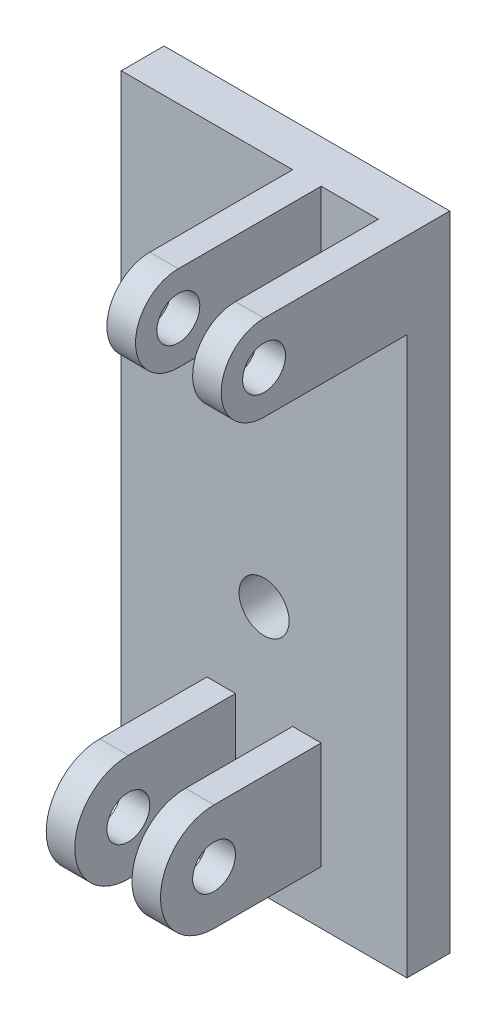
from build123d import *

# Parameters (mm, degrees)
SKETCH1_W           = 40
SKETCH1_H           = 90
BOSS_EXTRUDE1_DEPTH = 6
SKETCH3_R           = 3
BOSS_EXTRUDE2_DEPTH = 4
BOSS_EXTRUDE3_START = 4
SKETCH4_R           = 3
BOSS_EXTRUDE3_DEPTH = 4
LPATTERN1_COUNT     = 2
LPATTERN1_PITCH     = 12
SKETCH5_R           = 3.5
CUT_EXTRUDE1_DEPTH  = 56.686623169


with BuildPart() as part:
    # Sketch1 → Boss-Extrude1 (new body)
    with BuildSketch(Plane.XY):
        Rectangle(SKETCH1_W, SKETCH1_H)
    extrude(amount=BOSS_EXTRUDE1_DEPTH)

    # Sketch3 → Boss-Extrude2 (add)
    with BuildSketch(Plane.ZY.offset(-20)):
        with BuildLine():
            Line((26, 45), (6, 45))
            Line((6, 45), (6, 33))
            Line((6, 33), (26, 33))
            ThreePointArc((26, 33), (32, 39), (26, 45))
        make_face()
        with Locations(Location((26, 39, 0), (0, 0, 270))):
            Circle(SKETCH3_R, mode=Mode.SUBTRACT)
    boss_extrude2 = extrude(amount=BOSS_EXTRUDE2_DEPTH)

    # Sketch4 → Boss-Extrude3 (add)
    with BuildSketch(Plane(origin=(0, 0, 0), x_dir=(0, 0, -1), z_dir=(1, 0, 0)).offset(BOSS_EXTRUDE3_START)):
        with BuildLine():
            Line((-21, -22.5), (-6, -22.5))
            Line((-6, -22.5), (-6, -37.5))
            Line((-6, -37.5), (-21, -37.5))
            ThreePointArc((-21, -37.5), (-28.5, -30), (-21, -22.5))
        make_face()
        with Locations((-21, -30)):
            Circle(SKETCH4_R, mode=Mode.SUBTRACT)
    boss_extrude3 = extrude(amount=BOSS_EXTRUDE3_DEPTH)

    # Mirror1: Boss-Extrude3 across plane
    add(boss_extrude3.mirror(Plane(origin=(0, 0, 0), x_dir=(0, 0, 1), z_dir=(1, 0, 0))))

    # LPattern1: Boss-Extrude2 ×2
    with Locations(*[(-i * LPATTERN1_PITCH, 0, 0) for i in range(1, LPATTERN1_COUNT)]):
        add(boss_extrude2)

    # Sketch5 → Cut-Extrude1 (cut, through all)
    with BuildSketch(Plane.XY.offset(6)):
        with Locations((0, 20)):
            Circle(SKETCH5_R)
        with Locations((0, -10)):
            Circle(SKETCH5_R)
    extrude(amount=-CUT_EXTRUDE1_DEPTH, mode=Mode.SUBTRACT)


solid = part.part
